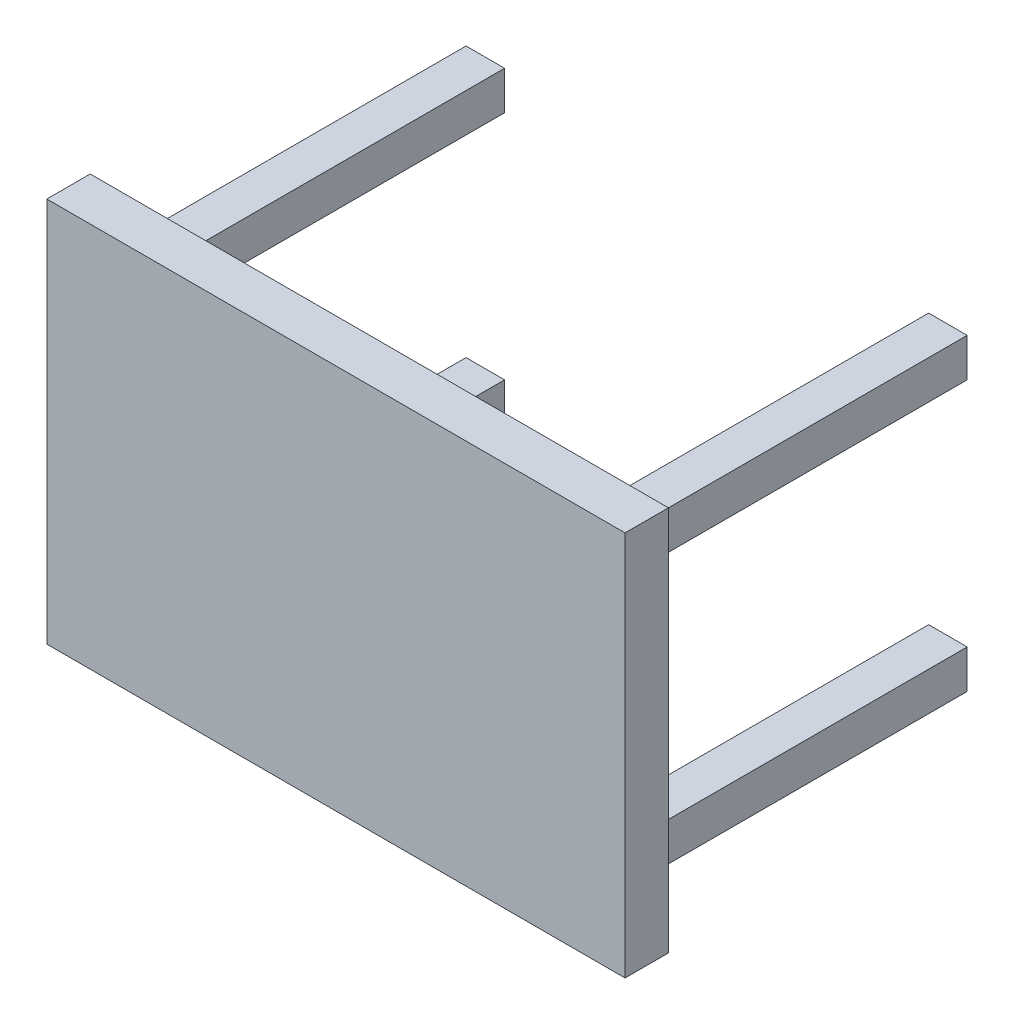
from build123d import *

# Parameters (mm, degrees)
SKETCH1_W               = 1200
SKETCH1_H               = 800
BOSS_EXTRUDE1_DEPTH     = 90
SKETCH2_W               = 80
SKETCH2_H               = 80
BOSS_EXTRUDE2_DEPTH     = 700
MIRROR2_COPY_1_SKETCH_W = 80
MIRROR2_COPY_1_SKETCH_H = 80
MIRROR2_COPY_1_DEPTH    = 700


with BuildPart() as part:
    # Sketch1 → Boss-Extrude1 (new body)
    with BuildSketch(Plane.XY):
        Rectangle(SKETCH1_W, SKETCH1_H)
    extrude(amount=-BOSS_EXTRUDE1_DEPTH)

    # Sketch2 → Boss-Extrude2 (add)
    with BuildSketch(Plane(origin=(0, 0, -90), x_dir=(-1, 0, 0), z_dir=(0, 0, -1))):
        with Locations((480, -280)):
            Rectangle(SKETCH2_W, SKETCH2_H)
    boss_extrude2 = extrude(amount=BOSS_EXTRUDE2_DEPTH)

    # Mirror1: Boss-Extrude2 across plane
    add(boss_extrude2.mirror(Plane.ZX))

    # Mirror2: Boss-Extrude2 across plane
    add(boss_extrude2.mirror(Plane(origin=(0, 0, 0), x_dir=(0, 0, 1), z_dir=(1, 0, 0))))

    # Mirror2 copy 1 sketch → Mirror2 copy 1 (add)
    with BuildSketch(Plane(origin=(0, 0, -90), x_dir=(1, 0, 0), z_dir=(0, 0, -1))):
        with Locations((480, -280)):
            Rectangle(MIRROR2_COPY_1_SKETCH_W, MIRROR2_COPY_1_SKETCH_H)
    extrude(amount=MIRROR2_COPY_1_DEPTH)


solid = part.part
